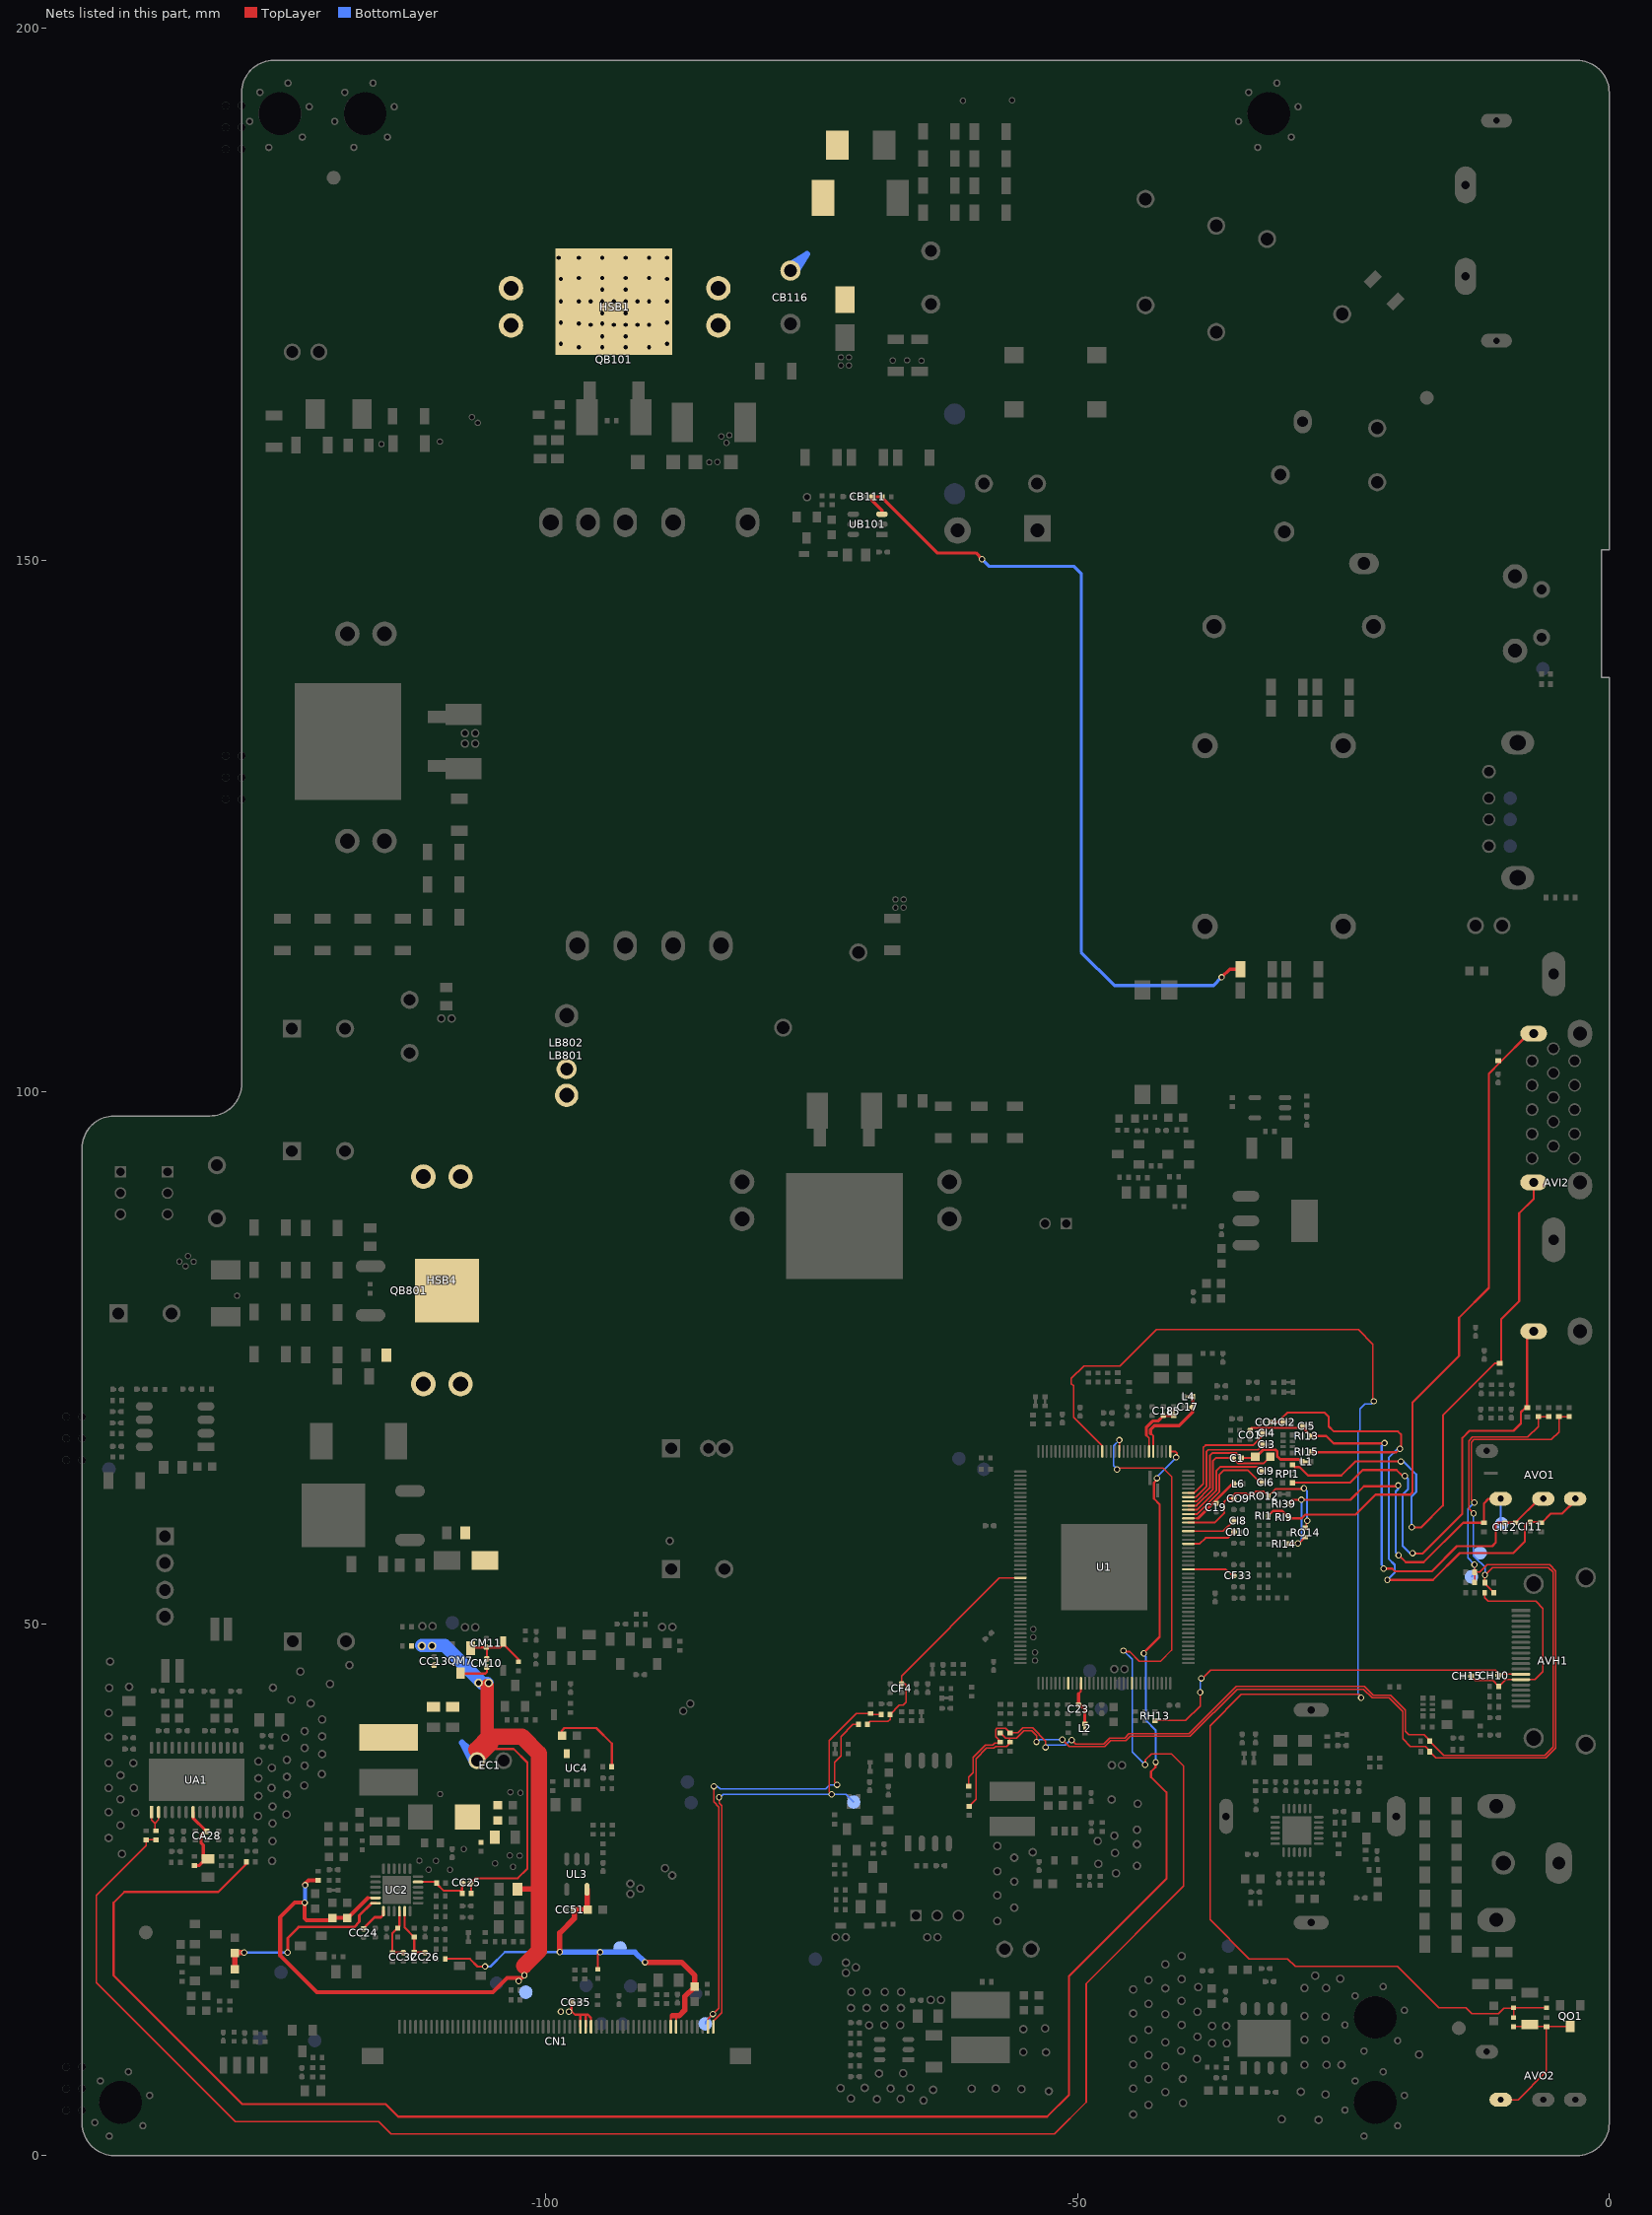
[diagram p0: the nets of this part, all layers, seen from the top]
# Altium PCB MISC86383-9.PcbDoc (part 8 of 18)
Units mm, origin at the board's own origin, x right, y up, seen from the top; angles counter-clockwise.
Board outline 143.6 x 197 mm, 2 copper layers (TopLayer, BottomLayer), stack 1.571 mm thick; 743 components, 401 nets, 2996 pads, 1077 vias.
Unrouted connection lines stored in the file: 4.

## Via types
v1: diameter 0.6, hole 0.4, TopLayer to BottomLayer, tented both sides, 993 vias
v2: diameter 0.6, hole 0.4, TopLayer to BottomLayer, 65 vias
v3: diameter 0.7, hole 0.5, TopLayer to BottomLayer, tented both sides, 15 vias
v4: diameter 0.8, hole 0.5, TopLayer to BottomLayer, tented both sides, 4 vias

## Nets (pads, with @x,y where several pads share a name; then routed paths per layer and width w, separated by ;. In a path a pad name is that pad's centre, name@x,y a point inside that pad or via, vN(x,y) a via of type N, cw(c..) or ccw(c..) an arc to the next point about the centre after c; other vN are vias at no path point) (continued)
AMP-MUTE: RA1.2 RA8.1 U1.59 | length 199.7
  TopLayer w0.127: U1.59@-46.071,66.213 v1(-46.071,67.265)
  TopLayer w0.152: RA8.1@-136.657,29.678 -136.664,29.684 RA1.2@-137.578,29.684 -137.578,29.138 -142.267,24.45 -142.267,16.257 -129.21,3.2 -115.722,3.2 -114.546,2.024 -52.18,2.024 -49.18,5.024 -49.18,16.174 -40.011,25.343 -40.011,36.633 -41.152,37.774 -43.049,37.774 -43.612,37.211 -43.612,36.843 -43.675,36.779 v1(-43.65,36.754) ; v1(-46.294,64.504) -46.144,64.655 -41.95,64.655 -41.154,63.859 -41.154,47.522 -42.186,46.489 -44.185,46.489 -45.079,47.383 -45.592,47.383 v1(-45.682,47.473)
  BottomLayer w0.152: v1(-46.294,64.504) -46.294,64.545 -46.62,64.87 -46.62,66.716 v1(-46.071,67.265) ; v1(-45.682,47.473) -44.856,46.647 -44.856,37.96 v1(-43.65,36.754)
AMP-RO: RA5.1 U1.47 | length 184.7
  TopLayer w0.178: U1.47@-41.271,66.213 -40.8,66.213 -40.653,66.065 -40.653,65.71 v1(-40.716,65.646)
  TopLayer w0.203: RA5.1@-128.153,27.602 -128.153,27.434 -130.797,24.79 -139.627,24.79 -140.641,23.776 -140.641,16.93 -128.536,4.826 -115.049,4.826 -113.873,3.65 -52.853,3.65 -50.805,5.697 -50.805,16.848 -41.637,26.016 -41.637,34.139 -43.086,35.588 -43.086,36.096 -42.672,36.511 v1@-42.672,36.991 ; v1@-43.764,47.282 -42.271,48.775 -42.271,61.22 -42.809,61.758 -42.809,63.269 v1@-42.524,63.554
  BottomLayer w0.203: v1(-43.764,47.206) -43.764,47.076 -43.561,46.873 -43.561,40.909 -42.644,39.991 v1(-42.644,36.991) ; v1@-42.585,63.752 v1@-40.716,65.621
  other v1: -42.524,63.69
AMP_STB/: RA8.2 UA1.1 UA1.2 | length 3.3
  TopLayer w0.152: UA1.1@-137.163,32.198 UA1.1@-137.07,32.291 -137.07,31.551 -136.758,31.24 -136.42,31.578 UA1.2@-136.42,32.291 ; -136.758,31.239 -136.758,30.629 RA8.2@-136.657,30.528
ARC: AVH1.14 CH15.1 DH3.K RH2.1 | length 20.2
  TopLayer w0.127: CH15.1@-13.123,45.072 CH15.1@-12.948,45.072 -12.948,45.028 -12.573,44.653 -10.937,44.653 DH3.K@-10.396,44.112 -10.211,44.298 -10.185,44.298 -9.733,44.75 AVH1.14@-8.3,44.75 -6.975,44.75 -6.223,45.502 -6.223,51.435 -6.909,52.121 -11.379,52.121 -11.702,52.444 RH2.1@-11.702,52.901
AU_VAG: C1.2@-35.41,65.586 C1.2@-35.235,65.586 C2.2 U1.38 | length 11.5
  TopLayer w0.178: U1.38@-39.571,61.113 -38.799,61.113 -37.256,62.655 -37.256,65.341 -37.012,65.586 C1.2@-35.41,65.586 ; C1.2@-35.323,65.499 -34.901,65.077 -32.512,65.077 -31.877,65.712 C2.2@-31.864,65.725
AU_VRM: C1.1 C2.1 L1.2 L1.3 U1.39 | length 15.6
  TopLayer w0.178: U1.39@-39.571,61.513 -38.83,61.513 -37.561,62.782 -37.561,65.811 -37.32,66.052 -35.026,66.052 C1.1@-34.56,65.586 -33.39,65.586 C2.1@-33.277,65.699
  TopLayer w0.254: C2.1@-33.277,65.699 -33.216,65.699 -32.562,66.353 -31.359,66.353 -31.21,66.205 -31.21,65.736 -30.928,65.453 -29.168,65.453 L1.2@-28.977,65.262
  TopLayer w0.305: L1.2@-28.977,65.262 -28.944,65.23 L1.2@-28.868,65.23
AV1_LIN: CI9.1 U1.37 | length 9.8
  TopLayer w0.178: U1.37@-39.571,60.713 -38.768,60.713 -36.952,62.529 -36.952,64.364 -36.555,64.76 -33.095,64.76 CI9.1@-32.692,64.357
AV1_RIN: CI6.1 U1.36 | length 10
  TopLayer w0.178: U1.36@-39.571,60.313 -38.737,60.313 -36.647,62.403 -36.647,64.039 -36.256,64.429 -33.962,64.429 -32.823,63.29 CI6.1@-32.692,63.29
AV2_LIN: CI4.1 U1.41 | length 11.4
  TopLayer w0.178: U1.41@-39.571,62.313 -39.021,62.313 -38.171,63.163 -38.171,66.573 -37.955,66.789 -33.474,66.789 -32.628,67.636 CI4.1@-32.628,67.935
AV2_RIN: CI3.1 U1.40 | length 10.9
  TopLayer w0.178: U1.40@-39.571,61.913 -38.862,61.913 -37.866,62.909 -37.866,66.218 -37.727,66.357 -33.043,66.357 CI3.1@-32.628,66.772
AV_L: AVI2.3 DI2.K RPI1.2 | length 55.9
  TopLayer w0.203: RPI1.2@-29.797,64.949 -29.575,64.728 -29.11,64.728 -28.324,63.942 -25.186,63.942 -23.858,65.269 -19.588,65.269 v1(-19.583,65.265) ; v1@-18.349,59.068 -17.679,59.068 -15.633,61.113 -15.633,69.617 -10.745,74.505 DI2.K@-10.274,74.505 -10.151,74.628 -10.151,78.644 -8.458,80.337 -8.458,88.602 -7.1,89.96 AVI2.3@-7.1,91.5
  BottomLayer w0.203: v1@-19.364,65.27 -18.148,64.054 -18.148,62.392 -18.593,61.948 -18.593,59.068 v1(-18.555,59.068)
AV_LIN/OUT: AVO1.4 CI5.2@-28.697,68.595 CI5.2@-28.872,68.595 CI12.1 CO1.1 DO1.K RI13.1 | length 44.7
  TopLayer w0.203: CO1.1@-33.853,68.194 -33.803,68.245 -33.618,68.43 -28.872,68.43 -28.793,68.43 RI13.1@-28.018,67.655 -26.614,67.655 -25.917,66.959 v1@-21.135,66.959 ; AVO1.4@-6.2,61.75 -6.576,61.75 -8.788,59.538 DO1.K@-8.788,59.505 CI12.1@-9.804,59.505 -10.51,59.505 -10.655,59.36 -10.655,57.633 -10.986,57.302 -14.317,57.302 -16.695,54.924 -20.142,54.924 -20.404,55.186 v1(-21.196,55.186) ; v1(-21.196,55.186) -21.226,55.156 -21.374,55.156 -21.345,55.186 v1(-21.196,55.186)
  BottomLayer w0.203: v1(-21.135,66.987) -21.395,66.728 -21.395,55.554 v1@-21.111,55.271
AV_R: AVI2.1 DI1.K RPI1.8 | length 48.5
  TopLayer w0.203: RPI1.8@-29.797,63.249 -29.764,63.282 -24.37,63.282 -23.186,64.465 -20.002,64.465 v1@-19.367,63.83 ; v1(-18.491,56.642) -18.542,56.591 -18.491,56.591 -17.569,56.591 -13.805,60.356 -13.805,67.478 -13.141,68.141 -9.002,68.141 -8.309,68.834 -8.309,69.907 -7.909,70.307 DI1.K@-7.717,70.307 -7.717,76.883 AVI2.1@-7.1,77.5
  BottomLayer w0.203: v1(-19.225,63.916) -19.342,64.033 -19.342,64.046 -19.218,63.922 -18.923,63.627 -18.923,62.65 -19.414,62.16 -19.414,57.295 -18.761,56.642 v1(-18.491,56.642)
AV_RIN/ROUT: AVO1.3 CI2.2@-30.531,68.963 CI2.2@-30.706,68.963 CI11.1 CO4.1 DO3.K RI15.1 | length 59.1
  TopLayer w0.203: CO4.1@-31.783,68.951 -30.718,68.951 CI2.2@-30.706,68.963 -30.706,69.415 -30.274,69.846 -26.746,69.846 -26.368,69.469 -26.368,68.564 -25.889,68.085 -19.85,68.085 -19.558,67.793 -19.558,66.586 v1(-19.693,66.451) -20.015,66.128 RI15.1@-28.018,66.128 ; v1(-20.861,54.119) -16.566,54.119 -14.043,56.642 -9.03,56.642 -7.925,57.747 -7.925,59.244 -7.613,59.556 CI11.1@-7.417,59.556 -6.451,59.556 DO3.K@-6.401,59.505 -6.331,59.505 -5.486,60.35 -4.42,60.35 -3.2,61.57 AVO1.3@-3.2,61.75
  BottomLayer w0.203: v1@-20.861,54.136 -20.168,54.83 -20.168,55.541 -20.734,56.108 -20.734,65.607 v1@-19.891,66.451
AVCC: CA28.2@-131.88,30.334 CA28.2@-131.88,30.509 RA3.2 RA4.2 UA1.7 | length 6.8
  TopLayer w0.305: UA1.7@-133.17,32.291 -133.17,31.752 CA28.2@-131.926,30.509 ; RA4.2@-133.048,27.271 -132.564,27.271 -131.933,27.902 RA3.2@-131.783,27.902 ; RA3.2@-132.203,27.936 -132.203,29.178 -132.409,29.384 -132.409,30.164 -132.065,30.509 CA28.2@-131.926,30.509 ; CA28.2@-131.88,30.509 CA28.2@-131.926,30.509
AVDD: AVDD.1 CC4.1 CC7.2 CC19.1 CC20.1 CC25.2@-107.024,25.645 CC25.2@-107.199,25.645 CC38.2 CG22.1 CG35.1 CN1.35 CN1.36 CN1.37 DC1.K EC1.1 pad.VIA5@-97.828,13.525 pad.VIA5@-98.59,13.525 pad.VIA5@-102.014,16.947 pad.VIA5@-102.552,16.408 pad.VIA5@-105.359,44.45 pad.VIA5@-106.324,44.45 pad.VIA5@-110.693,47.904 pad.VIA5@-111.658,47.904 RC1.1 RC18.2 RC19.2 RC31.1 RG8.2 RG15.2 UC2.5 UC4.5 | length 123.8
  TopLayer w0.203: -116.929,24.029 -116.735,24.223 UC2.5@-116.014,24.223 ; RG8.2@-107.019,24.632 -107.024,24.637 CC25.2@-107.024,25.645 -106.596,26.073 -102.641,26.073 -101.74,26.975 -101.74,36.944 -103.022,38.227 -105.365,38.227 ; CC38.2@-98.484,39.484 -98.484,39.873 -98.527,39.916 -98.254,40.189 -95.256,40.189 -93.796,38.729 RC31.1@-93.796,36.551 ; CG35.1@-97.593,14.402 -97.593,13.582 -97.25,13.24 -96.75,13.24 ; CN1.35@-96.75,12.103 -96.75,13.24 ; CN1.36@-96.25,12.103 -96.25,13.198 -96.291,13.24 ; CN1.37@-95.75,12.103 -95.75,12.946 -96.044,13.24 -96.291,13.24 ; -96.75,13.24 -96.291,13.24
  TopLayer w0.381: v1@-122.714,25.496 -122.329,25.882 RG15.2@-121.405,25.882 ; -116.735,24.203 -116.742,24.203 -118.6,22.344 CC4.1@-118.681,22.344 CC7.2@-120.053,22.344 -120.287,22.111 -122.504,22.111 -122.682,22.288 v1(-122.682,23.787) -123.597,23.787 -124.982,22.402 -124.982,18.81 -121.514,15.342 -104.975,15.342 -103.629,16.688 -102.552,16.688 -102.273,16.688
  TopLayer w0.508: RC1.1@-102.664,25.044 -100.698,25.044 ; -100.698,25.197 -100.647,25.248
  TopLayer w1.016: EC1.1@-106.47,37.122 -105.365,38.227 -104.959,38.633 -104.959,39.395
  TopLayer w1.27: pad.VIA5@-105.512,44.196 -105.512,39.573 -105.334,39.395
  TopLayer w1.524: -106.54,38.189 -105.334,39.395 -104.959,39.395 -102.248,39.395 -100.647,37.795 -100.647,25.248 -100.647,19.247 -102.052,17.842
  BottomLayer w0.381: v1(-122.682,23.787) -122.631,23.838 v1(-122.631,25.413)
  BottomLayer w1.27: pad.VIA5@-111.658,47.95 -110.693,47.95 -109.506,47.95 -106.165,44.609 -105.955,44.399 pad.VIA5@-105.512,44.399
AVDD5V_MHL: U1.147
AVDD_AU33: C19.2@-36.944,61.36 C19.2@-36.944,61.185 L6.2 L6.3 U1.35 | length 5.6
  TopLayer w0.178: U1.35@-39.571,59.913 -38.773,59.913
  TopLayer w0.254: -38.773,59.913 -38.652,59.913 -35.395,63.17 L6.2@-35.299,63.17
AVDD_DADC: C17.2@-39.161,70.371 C17.2@-39.336,70.371 L4.2 L4.3 U1.51 | length 8.2
  TopLayer w0.178: -43.059,67.824 -42.871,67.636 U1.51@-42.871,66.213
  TopLayer w0.305: -43.123,67.898 -43.123,68.278 -42.766,68.635 -40.439,68.635 -39.161,69.913 C17.2@-39.161,70.371 -39.161,71.361 L4.2@-39.148,71.374
AVDD_DMPLL: C18.2@-41.912,69.577 C18.2@-41.912,69.752 L5.2 L5.3 U1.52 | length 5.4
  TopLayer w0.178: -43.542,67.729 -43.271,67.458 U1.52@-43.271,66.213
  TopLayer w0.279: -43.542,67.729 -43.542,68.452 -42.939,69.054 -42.435,69.054 C18.2@-41.912,69.577
  TopLayer w0.305: C18.2@-41.912,69.577 -40.972,69.577 L5.2@-40.959,69.564
AVDD_FB: CC25.1 RG8.1 RG13.2 UC2.17 | length 5.3
  TopLayer w0.203: UC2.17@-112.014,25.723 -110.37,25.723 RG13.2@-110.264,25.618 -110.264,25.555 -109.601,24.892 -107.874,24.892 CC25.1@-107.874,25.645
AVDD_MOS_G: CM10.2@-105.55,46.554 CM10.2@-105.55,46.729 CM11.1 DM3.K QM7.G RM12.2 | length 6.6
  TopLayer w0.203: QM7.G@-107.063,47.961 -106.936,47.834 -106.874,47.772 CM11.1@-105.588,47.772 -104.273,47.772 -103.988,48.057 DM3.K@-103.988,48.327 ; CM10.2@-105.55,46.691 CM10.2@-105.55,46.729 CM11.1@-105.55,47.695 ; DM3.K@-103.829,47.924 -102.565,46.66 RM12.2@-102.565,46.424
AVDD_SOURCE_IN: CC8.2 CC12.2 CC13.2@-110.503,46.07 CC13.2@-110.503,46.245 CM10.1 LC1.1 QM7.D | length 3.1
  TopLayer w0.203: QM7.D@-108.013,45.357 -107.97,45.314 -105.664,45.314 -105.55,45.428 CM10.1@-105.55,45.879 CM10.1@-105.55,46.032
BANK_SEL_IC: U1.132
BRO: CB111.1 RB104.2 RB142.1 UB101.3 | length 77.5
  TopLayer w0.3: UB101.3@-68.386,154.341 -68.386,154.708 -69.311,155.633 CB111.1@-69.311,155.994 -69.285,155.969 RB104.2@-68.357,155.969 -68.357,155.86 -63.188,150.691 -59.556,150.691 v2(-58.979,150.114) ; v2(-36.436,110.787) -35.68,111.544 RB142.1@-34.672,111.544
  BottomLayer w0.3: v2(-58.979,150.114) -58.289,149.424 -57.493,149.424 ; -57.751,149.424 -57.493,149.424 ; v2(-36.436,110.787) -37.208,110.015 -46.528,110.015 -49.652,113.139 -49.652,148.766 -50.309,149.424 -57.493,149.424
CEC: AVH1.13 CH10.2@-10.57,45.148 CH10.2@-10.395,45.148 RH13.1 | length 38.4
  TopLayer w0.127: RH13.1@-42.714,40.892 -39.826,40.892 -38.468,42.25 v1(-38.468,43.548) ; v1(-38.363,44.874) -38.363,44.739 -38.296,44.806 -37.469,45.634 -10.697,45.634 -10.395,45.332 CH10.2@-10.395,45.28 ; CH10.2@-10.395,45.148 CH10.2@-10.395,45.28 ; AVH1.13@-8.3,45.25 -10.365,45.25 CH10.2@-10.395,45.28
  BottomLayer w0.127: v1(-38.468,43.548) -38.468,44.769 v1(-38.363,44.874)
CPV: CN1.60 CPV.1 RG25.2 RG62.2 | length 45.9
  TopLayer w0.127: CN1.60@-84.25,12.103 -84.25,12.626 -83.464,13.412 -83.464,32.88 -83.706,33.122 v1(-83.706,33.68) ; -73.368,34.163 -73.368,39.002 -70.808,41.561 RG62.2@-69.469,41.561 -69.386,41.478 RG25.2@-68.472,41.478
  BottomLayer w0.127: v1(-83.706,33.68) -83.617,33.68 -83.325,33.972 v1(-73.127,33.972) -71.78,33.972 CPV.1@-71.044,33.236
CPV2: CN1.59 CPV2.1 RG59.2 | length 43
  TopLayer w0.127: CN1.59@-84.75,12.103 -84.75,12.837 v1(-84.277,13.31) -83.718,13.869 -83.718,32.775 -84.196,33.253 -84.196,34.409 ; v1(-72.619,34.861) -72.86,35.103 -72.86,36.957 -72.259,37.558 -72.259,39.392 -71.113,40.538 RG59.2@-70.605,40.538
  BottomLayer w0.127: CPV2.1@-85.001,12.383 -85.001,12.548 -84.277,13.271 v1(-84.277,13.31) ; v1(-84.201,34.722) -83.849,34.722 -83.608,34.48 -73.671,34.48 -73.29,34.861 v1(-72.619,34.861)
CPV/: CF4.1 RG25.1 RG59.1 U1.104 | length 22.6
  TopLayer w0.127: RG59.1@-69.755,40.538 -69.484,40.809 -67.827,40.809 -67.622,41.014 RG25.1@-67.622,41.478 -67.615,41.478 -66.751,42.342 -66.402,42.342 -66.108,42.636 -66.108,44.264 -66.211,44.367 CF4.1@-66.548,44.367 -66.548,45.103 -57.338,54.313 U1.104@-55.371,54.313
CVBS_IN: CI8.1 U1.32 | length 4.7
  TopLayer w0.178: U1.32@-39.571,58.713 -36.3,58.713 CI8.1@-35.307,59.705
CVBS_IN/: AVI2.5 DI3.K RI1.1 RI9.2 | length 63.2
  TopLayer w0.203: RI1.1@-32.057,60.162 -31.611,60.608 -30.736,60.608 -30.151,60.023 -30.049,59.921 -28.924,59.921 -28.585,60.26 -23.86,60.26 -21.979,62.141 -18.704,62.141 -18.496,62.349 -18.496,70.802 -14.117,75.181 -14.117,78.782 -11.321,81.578 -11.321,101.735 -10.277,102.778 -7.555,105.5 AVI2.5@-7.1,105.5
CVBS_IN/OUT: AVO1.2 CVBS_IN/OUT.1 DO2.K RI14.1 RI39.1 RO14.1 | length 40
  TopLayer w0.203: RI39.1@-30.152,61.28 -29.771,61.661 -29.223,61.661 -29.208,61.646 -28.939,61.646 -24.337,61.646 -23.062,62.92 v1@-19.871,62.92 ; RI14.1@-30.141,57.495 -30.078,57.559 v1(-29.269,57.559) ; v1@-29.228,57.518 RO14.1@-28.596,58.15 ; v1(-19.842,63) -19.842,62.949 v1@-19.871,62.92 ; v1(-19.796,56.443) -19.136,55.783 -17.444,55.783 -13.721,59.505 DO2.K@-11.786,59.505 -11.786,61.316 -11.351,61.75 AVO1.2@-10.2,61.75 ; v1@-19.668,62.92 -19.842,62.92 v1@-19.871,62.92
  BottomLayer w0.203: v1@-29.256,57.546 -28.939,57.864 v1(-28.939,61.661) v1@-28.939,61.807 ; v1(-19.842,63) -19.842,62.665 -20.074,62.433 -20.074,56.721 v1(-19.796,56.443) ; AVO1.2@-10.2,61.75 -10.2,59.491 CVBS_IN/OUT.1@-10.108,59.398
CVBS_OUT: CO9.2@-35.132,61.788 CO9.2@-35.307,61.788 RO12.1 RO14.2 U1.34 | length 17.3
  TopLayer w0.178: U1.34@-39.571,59.513 -37.096,59.513 -36.182,60.427 -36.182,61.481 -35.875,61.788 CO9.2@-35.307,61.788 -35.307,62.127 -35.155,62.279 -34.132,62.279 -33.997,62.143 -33.535,62.143 -33.221,62.457 -32.523,62.457 RO12.1@-32.057,61.991 -31.388,62.66 -28.851,62.66 -28.728,62.783 v1(-28.697,62.753) ; RO14.2@-28.596,59 -28.481,59.114 v1@-28.481,59.616
  BottomLayer w0.203: v1@-28.596,62.651 -28.405,62.461 v1(-28.405,59.692)
D_QB101: BB101.1 CB116.2 DB106.A DB107.A HSB1.1 HSB1.2 HSB1.3 HSB1.4 QB101.2
  other v1: -96.888,170.048 -94.688,170.048 -92.488,170.048 -90.288,170.048 -98.588,170.348 -88.588,170.348 -94.688,171.048 -92.488,171.048 -95.788,172.148 -93.588,172.148 -92.488,172.148 -91.388,172.148 -90.288,172.148 -96.888,172.248 -94.688,172.248 -98.588,172.348 -88.588,172.348 -94.688,173.248 -92.488,173.248 -98.588,174.348 -96.888,174.348 -95.788,174.348 -94.688,174.348 -93.588,174.348 -92.488,174.348 -91.388,174.348 -90.288,174.348 -88.588,174.348 -94.688,175.448 -92.488,175.448 -98.588,176.448 -88.588,176.448 -96.888,176.548 -94.688,176.548 -92.488,176.548 -90.288,176.548 -98.788,178.448 -96.888,178.448 -94.688,178.448 -92.488,178.448 -90.288,178.448 -88.588,178.448
D_QB801: BB801.1 BB802.1 CB809.2 HSB4.1 HSB4.2 HSB4.3 HSB4.4 LB801.2 LB802.2 QB801.D
DDC_SCL/UART_RX: DV3.K DV6.K DV7.K RH2.2 RV13.1 RV19.2 RV21.2 RV22.1 UART_RX.1 | length 116
  TopLayer w0.127: RV21.2@-60.223,34.715 -60.223,35.573 -59.804,35.992 -59.804,37.423 -58.645,38.583 -57.976,38.583 -57.779,38.78 -57.378,38.78 RV13.1@-57.277,38.881 ; RV13.1@-57.213,38.89 -57.24,38.917 -57.702,39.379 -57.702,40.041 -57.591,40.152 -56.763,40.152 RV19.2@-56.348,39.737 -55.608,39.737 -55.132,40.212 -54.218,40.212 -52.995,38.99 v1(-52.995,38.384) ; v1(-50.557,39.069) -50.189,38.701 -47.55,38.701 -46.987,39.265 -45.552,39.265 -45.151,39.666 -39.521,39.666 -35.078,44.11 -22.998,44.11 -22.174,43.285 -20.561,43.285 -19.164,41.888 -19.164,39.908 -18.826,39.571 -17.397,39.571 -16.881,39.054 DV7.K@-16.881,38.969 -15.535,37.623 -6.07,37.623 -5.283,38.41 -5.283,54.866 -5.713,55.296 -10.976,55.296 v1(-11.684,54.588) -11.685,54.587 DV3.K@-11.685,53.861 ; v1@-12.789,60.338 -12.687,60.236 -12.687,60.312 v1(-12.751,60.376) -13.208,60.833 -13.208,67.184 -12.847,67.544 -7.657,67.544 -6.655,68.546 DV6.K@-6.655,69.476 RV22.1@-5.69,69.476 ; DV3.K@-11.612,53.693 -10.836,52.917 RH2.2@-10.813,52.894
  BottomLayer w0.127: v1(-52.995,38.384) -53.046,38.434 -52.863,38.617 -51.159,38.617 -50.706,39.069 v1(-50.557,39.069) ; v1(-12.751,60.376) -12.751,56.667 -12.751,56.401 -12.576,56.226 -11.684,55.334 v1(-11.684,54.588)
DDC_SDA/UART_TX: DV4.K DV5.K DV8.K RH1.2 RV12.1 RV18.2 RV20.2 RV23.1 UART_TX.1 | length 120.3
  TopLayer w0.127: RV20.2@-60.401,32.81 RV20.2@-60.401,32.817 ; RV20.2@-60.198,32.835 -59.55,33.483 -59.55,37.318 -58.565,38.303 -57.861,38.303 -57.699,38.465 -56.683,38.465 -56.35,38.798 RV12.1@-56.35,38.881 ; RV18.2@-57.262,39.737 -56.773,39.247 -56.363,39.247 ; RV12.1@-56.333,38.89 -56.337,38.894 -56.363,38.92 -56.363,39.247 ; v1(-53.858,38.892) -53.858,39.494 -54.305,39.941 -55.044,39.941 -55.738,39.247 -56.363,39.247 ; v1(-51.421,39.107) -50.76,38.447 -47.445,38.447 -46.891,39.002 -45.456,39.002 -45.045,39.412 -39.416,39.412 -34.973,43.856 -23.104,43.856 -22.279,43.031 -20.697,43.031 -19.449,41.783 -19.418,41.783 -19.418,39.194 -18.704,38.479 -17.289,38.479 -16.865,38.055 DV8.K@-16.865,37.952 -16.282,37.369 -5.965,37.369 -5.029,38.305 -5.029,54.978 -5.601,55.55 -11.468,55.55 -12.171,54.847 DV4.K@-12.649,54.847 ; v1(-12.687,61.404) -12.979,61.696 -12.979,67.049 -12.712,67.315 -5.43,67.315 -4.724,68.021 DV5.K@-4.724,69.476 RV23.1@-3.759,69.476 ; v1(-12.661,55.574) -12.661,55.457 -12.649,55.444 DV4.K@-12.649,54.847 ; RH1.2@-12.649,53.882 DV4.K@-12.649,54.847
  BottomLayer w0.127: v1@-53.655,38.993 -53.541,39.107 v1(-51.421,39.107) ; UART_TX.1@-12.954,54.419 -12.661,54.712 v1(-12.661,55.574) -13.297,56.21 -13.297,60.811 v1@-12.84,61.268
DRVN: CC24.1 UC2.7 | length 2.7
  TopLayer w0.254: CC24.1@-117.129,21.362 -116.1,22.391 -115.506,22.391 -115.264,22.634 UC2.7@-115.264,22.973
DRVP: CC27.2 CC31.2 UC2.6 | length 17.8
  TopLayer w0.254: v1(-124.269,19.088) -124.269,20.46 -123.241,21.488 -118.021,21.488 -117.538,21.971 -117.538,22.568 -116.383,23.723 UC2.6@-116.014,23.723
  TopLayer w0.508: CC31.2@-129.235,17.521 CC27.2@-129.235,19.055 -129.202,19.088 v1(-128.359,19.088)
  BottomLayer w0.254: v1(-128.359,19.088) v1(-124.269,19.088)
DVDD: CC50.1 CC51.2@-97.314,23.114 CC51.2@-97.489,23.114 CG31.2 CN1.52 CN1.53 DVDD.1 RG7.2 RG49.2 UL3.5 | length 42.3
  TopLayer w0.203: RG49.2@-109.455,18.466 -109.43,18.491 -107.137,18.491 -106.413,17.767 v1(-105.715,17.767) v1@-105.689,17.767 ; RG7.2@-95.11,17.507 -95.11,18.885 v1(-94.882,19.113) ; CN1.52@-88.25,12.103 -88.25,12.969 -88.087,13.132 ; -87.833,13.132 -87.75,13.049 CN1.53@-87.75,12.103
  TopLayer w0.508: v1(-98.679,19.126) -98.679,20.917 -97.314,22.282 CC51.2@-97.314,23.114 CC50.1@-96.058,23.114 -96.116,23.172 UL3.5@-96.116,25.029 ; v1(-90.665,18.174) -87.247,18.174 -85.992,16.918 CG31.2@-85.992,15.883 -86.931,14.943 -86.931,13.662 -87.461,13.132 -87.833,13.132 ; -88.087,13.132 -87.833,13.132 ; -87.461,13.134 -87.831,13.134 -87.833,13.132
  BottomLayer w0.203: v1(-105.715,17.767) -105.207,17.767 -103.848,19.126 v1(-98.679,19.126)
  BottomLayer w0.508: v1(-98.679,19.126) -94.882,19.126 -93.015,19.126 -91.618,19.126 v1(-90.665,18.174)
DVDD_DDR: C23.2@-49.909,42.228 C23.2@-49.909,42.403 L2.2 L2.3 U1.135 | length 4.3
  TopLayer w0.178: -49.909,43.413 -49.671,43.651 U1.135@-49.671,44.413
  TopLayer w0.305: -49.909,43.413 -49.909,42.39 -49.763,42.39 -49.312,41.94 L2.2@-49.312,40.587
EXE_IR: RO6.2 RO9.2 RO10.2 U1.63 | length 143.4
  TopLayer w0.127: U1.63@-47.671,66.213 -47.671,66.741 -50.365,69.435 -50.365,72.372 -50.569,72.576 -50.569,73.075 -49.409,74.236 -46.007,74.236 -42.593,77.65 -23.574,77.65 -22.22,76.297 v1@-22.22,71.08 ; v1(-23.32,43.055) -23.259,43.117 -23.515,43.373 -34.587,43.373 -37.535,40.426 -37.535,22.185 -33.854,18.504 -30.238,18.504 -29.502,17.767 -19.904,17.767 -16.033,13.896 -13.462,13.896 -12.901,13.335 -10.41,13.335 -9.898,13.847 -9.04,13.847 RO6.2@-8.992,13.896 ; RO9.2@-8.992,12.968 RO6.2@-8.992,13.896 ; RO10.2@-5.893,13.896 RO6.2@-8.992,13.896
  BottomLayer w0.127: v1(-23.32,43.055) -23.613,43.349 -23.613,67.098 -23.613,68.036 -23.439,68.21 -23.439,70.196 -22.948,70.688 -22.365,70.688 v1(-22.128,70.924)
EXT_IRO: AVO2.2 DI5.K QO1.C RO2.1 RO9.1 | length 14.9
  TopLayer w0.127: AVO2.2@-10.2,5.25 -8.568,5.25 -5.893,7.925 DI5.K@-5.893,12.118 ; RO9.1@-8.992,12.118 -7.468,12.118 -7.308,12.118 -7.29,12.136 -5.893,12.136 QO1.C@-3.67,12.136
FBN: CC26.1 RG21.1 RG22.2 UC2.11 | length 5.3
  TopLayer w0.203: UC2.11@-113.264,22.973 -113.264,21.418 RG22.2@-112.376,20.53 RG21.1@-112.376,19.094 CC26.1@-111.36,19.094
FBP: CC32.1 RG9.1 RG14.2 UC2.10 | length 5
  TopLayer w0.203: RG9.1@-114.399,19.089 -114.442,19.132 -114.442,20.9 -113.944,21.398 -113.764,21.578 UC2.10@-113.764,22.973 ; RG9.1@-114.357,19.094 -113.567,19.094 CC32.1@-113.54,19.067
GIN0M: CF33.1 U1.23 | length 4.5
  TopLayer w0.152: U1.23@-39.571,55.113 -36.025,55.113 -35.435,54.523 CF33.1@-35.316,54.523
GIN1M: CI10.1 U1.29 | length 4.7
  TopLayer w0.178: U1.29@-39.571,57.513 -38.525,57.513 -37.96,58.077 -35.865,58.077 -35.307,58.635 CI10.1@-35.307,58.638